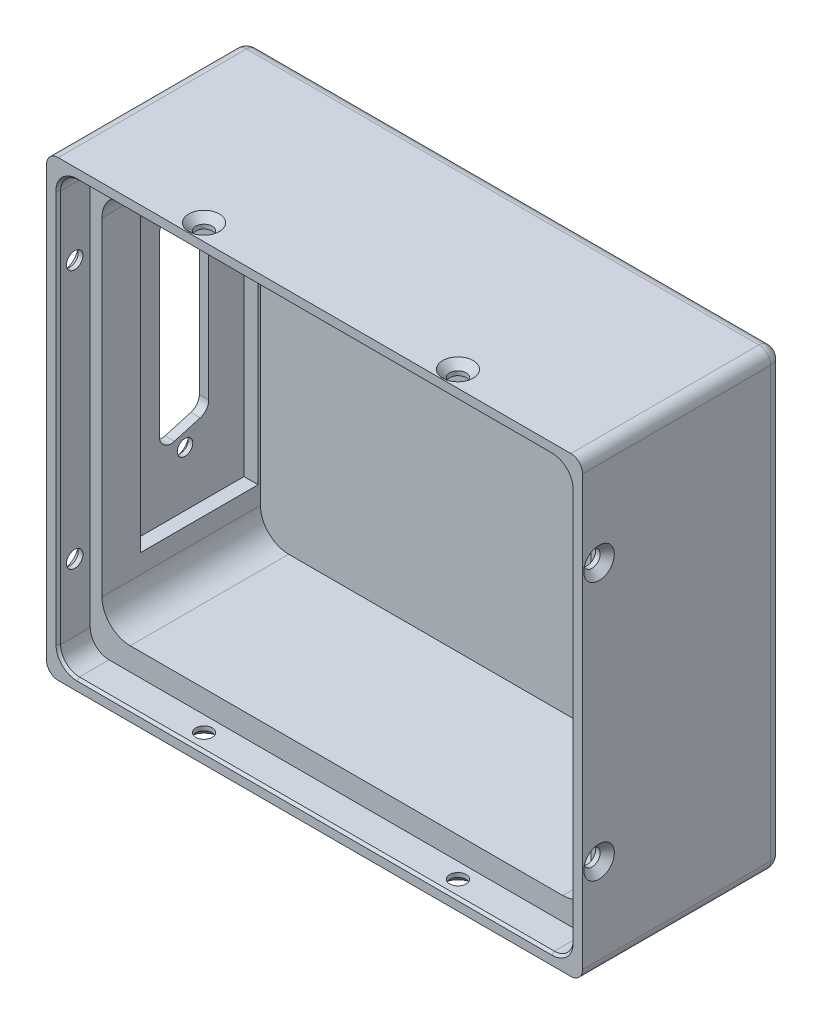
from build123d import *

# Parameters (mm, degrees)
SKETCH_1_W                  = 114
SKETCH_1_H                  = 96.3
EXTRUDE_1_DEPTH             = 42.5
SKETCH_2_W                  = 104
SKETCH_2_H                  = 81.8
CUT_EXTRUDE_1_DEPTH         = 40.5
SKETCH_3_W                  = 109
SKETCH_3_H                  = 91.5
CUT_EXTRUDE_2_DEPTH         = 6.8
FILLET_1_R                  = 2.5
FILLET_2_R                  = 4
FILLET_3_R                  = 6
HOLE_WIZARD_1_D             = 3.5
HOLE_WIZARD_1_DEPTH         = 10
HOLE_WIZARD_1_CSINK_D       = 6.5
HOLE_WIZARD_1_CSINK_ANGLE   = 90
PATTERN_LINEAR_1_COUNT      = 2
PATTERN_LINEAR_1_PITCH      = 54
MIRROR_1_COPY_1_D           = 3.5
MIRROR_1_COPY_1_DEPTH       = 10
MIRROR_1_COPY_1_CSINK_D     = 6.5
MIRROR_1_COPY_1_CSINK_ANGLE = 90
HOLE_WIZARD_2_D             = 3.5
HOLE_WIZARD_2_DEPTH         = 10
HOLE_WIZARD_2_CSINK_D       = 6.5
HOLE_WIZARD_2_CSINK_ANGLE   = 90
PATTERN_LINEAR_2_COUNT      = 2
PATTERN_LINEAR_2_PITCH      = 55
MIRROR_2_COPY_1_D           = 3.5
MIRROR_2_COPY_1_DEPTH       = 10
MIRROR_2_COPY_1_CSINK_D     = 6.5
MIRROR_2_COPY_1_CSINK_ANGLE = 90
CUT_EXTRUDE_3_DEPTH         = 6.8
FILLET_4_R                  = 2.5
SKETCH_8_W                  = 25
SKETCH_8_H                  = 70
CUT_EXTRUDE_4_DEPTH         = 3
HOLE_WIZARD_3_D             = 3.3
HOLE_WIZARD_3_DEPTH         = 10
HOLE_WIZARD_3_CBORE_D       = 5.5
HOLE_WIZARD_3_CBORE_DEPTH   = 1
PATTERN_LINEAR_3_COUNT      = 2
PATTERN_LINEAR_3_PITCH      = 47
CHAMFER_1_SIZE              = 0.5


with BuildPart() as part:
    # 草图1 → 拉伸1 (new body)
    with BuildSketch(Plane.XY):
        Rectangle(SKETCH_1_W, SKETCH_1_H)
    extrude(amount=EXTRUDE_1_DEPTH)

    # 草图2 → 切除-拉伸1 (cut)
    with BuildSketch(Plane.XY.offset(42.5)):
        Rectangle(SKETCH_2_W, SKETCH_2_H)
    extrude(amount=-CUT_EXTRUDE_1_DEPTH, mode=Mode.SUBTRACT)

    # 草图3 → 切除-拉伸2 (cut)
    with BuildSketch(Plane.XY.offset(42.5)):
        Rectangle(SKETCH_3_W, SKETCH_3_H)
    extrude(amount=-CUT_EXTRUDE_2_DEPTH, mode=Mode.SUBTRACT)

    # 圆角1
    fillet_1_edges = [part.edges().sort_by_distance(p)[0] for p in [
        (0, 48.15, 0),
        (57, 0, 0),
        (0, -48.15, 0),
        (-57, 0, 0),
        (-57, 48.15, 21.25),
        (57, 48.15, 21.25),
        (57, -48.15, 21.25),
        (-57, -48.15, 21.25),
    ]]
    fillet(fillet_1_edges, radius=FILLET_1_R)

    # 圆角2
    fillet_2_edges = [part.edges().sort_by_distance(p)[0] for p in [
        (-54.5, -45.75, 39.1),
        (-54.5, 45.75, 39.1),
        (54.5, 45.75, 39.1),
        (54.5, -45.75, 39.1),
    ]]
    fillet(fillet_2_edges, radius=FILLET_2_R)

    # 圆角3
    fillet_3_edges = [part.edges().sort_by_distance(p)[0] for p in [
        (-52, -40.9, 18.85),
        (-52, 40.9, 18.85),
        (52, 40.9, 18.85),
        (52, -40.9, 18.85),
    ]]
    fillet(fillet_3_edges, radius=FILLET_3_R)

    # 孔1
    with Locations(Plane(origin=(27, 48.15, 39), x_dir=(0, 0, 1), z_dir=(0, 1, 0))):
        with Locations((0, 0)):
            hole_wizard_1 = CounterSinkHole(HOLE_WIZARD_1_D / 2, HOLE_WIZARD_1_CSINK_D / 2, depth=HOLE_WIZARD_1_DEPTH, counter_sink_angle=HOLE_WIZARD_1_CSINK_ANGLE)

    # 阵列(线性)1: 孔1 ×2
    with Locations(*[(-i * PATTERN_LINEAR_1_PITCH, 0, 0) for i in range(1, PATTERN_LINEAR_1_COUNT)]):
        add(hole_wizard_1, mode=Mode.SUBTRACT)

    # 镜向1: 孔1 across plane
    add(hole_wizard_1.mirror(Plane.ZX), mode=Mode.SUBTRACT)

    # 镜向1 copy 1
    with Locations(Plane(origin=(-27, -48.15, 39), x_dir=(0, 0, 1), z_dir=(0, -1, 0))):
        with Locations((0, 0)):
            CounterSinkHole(MIRROR_1_COPY_1_D / 2, MIRROR_1_COPY_1_CSINK_D / 2, depth=MIRROR_1_COPY_1_DEPTH, counter_sink_angle=MIRROR_1_COPY_1_CSINK_ANGLE)

    # 孔2
    with Locations(Plane(origin=(-57, 27.5, 39), x_dir=(0, -1, 0), z_dir=(-1, 0, 0))):
        with Locations((0, 0)):
            hole_wizard_2 = CounterSinkHole(HOLE_WIZARD_2_D / 2, HOLE_WIZARD_2_CSINK_D / 2, depth=HOLE_WIZARD_2_DEPTH, counter_sink_angle=HOLE_WIZARD_2_CSINK_ANGLE)

    # 阵列(线性)2: 孔2 ×2
    with Locations(*[(0, -i * PATTERN_LINEAR_2_PITCH, 0) for i in range(1, PATTERN_LINEAR_2_COUNT)]):
        add(hole_wizard_2, mode=Mode.SUBTRACT)

    # 镜向2: 孔2 across plane
    add(hole_wizard_2.mirror(Plane(origin=(0, 0, 0), x_dir=(0, 0, 1), z_dir=(1, 0, 0))), mode=Mode.SUBTRACT)

    # 镜向2 copy 1
    with Locations(Plane(origin=(57, -27.5, 39), x_dir=(0, -1, 0), z_dir=(1, 0, 0))):
        with Locations((0, 0)):
            CounterSinkHole(MIRROR_2_COPY_1_D / 2, MIRROR_2_COPY_1_CSINK_D / 2, depth=MIRROR_2_COPY_1_DEPTH, counter_sink_angle=MIRROR_2_COPY_1_CSINK_ANGLE)

    # 草图7 → 切除-拉伸3 (cut)
    with BuildSketch(Plane.ZY.offset(57)):
        Polygon((10, 23.15), (10, -14.85), (20.5, -17.85), (20.5, 26.15), align=None)
    extrude(amount=-CUT_EXTRUDE_3_DEPTH, mode=Mode.SUBTRACT)

    # 圆角4
    fillet_4_edges = [part.edges().sort_by_distance(p)[0] for p in [
        (-54.5, 23.15, 10),
        (-54.5, 26.15, 20.5),
        (-54.5, -17.85, 20.5),
        (-54.5, -14.85, 10),
    ]]
    fillet(fillet_4_edges, radius=FILLET_4_R)

    # 草图8 → 切除-拉伸4 (cut, symmetric)
    with BuildSketch(Plane(origin=(-52, 0, 0), x_dir=(0, 0, -1), z_dir=(1, 0, 0))):
        with Locations((-15, 4.15)):
            Rectangle(SKETCH_8_W, SKETCH_8_H)
    extrude(amount=CUT_EXTRUDE_4_DEPTH, both=True, mode=Mode.SUBTRACT)

    # 孔3
    with Locations(Plane(origin=(-57, 27.803010051, 15.043686383), x_dir=(0, -1, 0), z_dir=(-1, 0, 0))):
        with Locations((0, 0)):
            hole_wizard_3 = CounterBoreHole(HOLE_WIZARD_3_D / 2, HOLE_WIZARD_3_CBORE_D / 2, HOLE_WIZARD_3_CBORE_DEPTH, depth=HOLE_WIZARD_3_DEPTH)

    # 阵列(线性)3: 孔3 ×2
    with Locations(*[(0, -i * PATTERN_LINEAR_3_PITCH, 0) for i in range(1, PATTERN_LINEAR_3_COUNT)]):
        add(hole_wizard_3, mode=Mode.SUBTRACT)

    # 倒角1
    chamfer_1_edges = [part.edges().sort_by_distance(p)[0] for p in [
        (0, 45.75, 42.5),
        (54.5, 0, 42.5),
        (-54.5, 0, 42.5),
        (0, -45.75, 42.5),
        (53.328427125, 44.578427125, 42.5),
        (-53.328427125, 44.578427125, 42.5),
        (-53.328427125, -44.578427125, 42.5),
        (53.328427125, -44.578427125, 42.5),
    ]]
    chamfer(chamfer_1_edges, length=CHAMFER_1_SIZE)


solid = part.part
